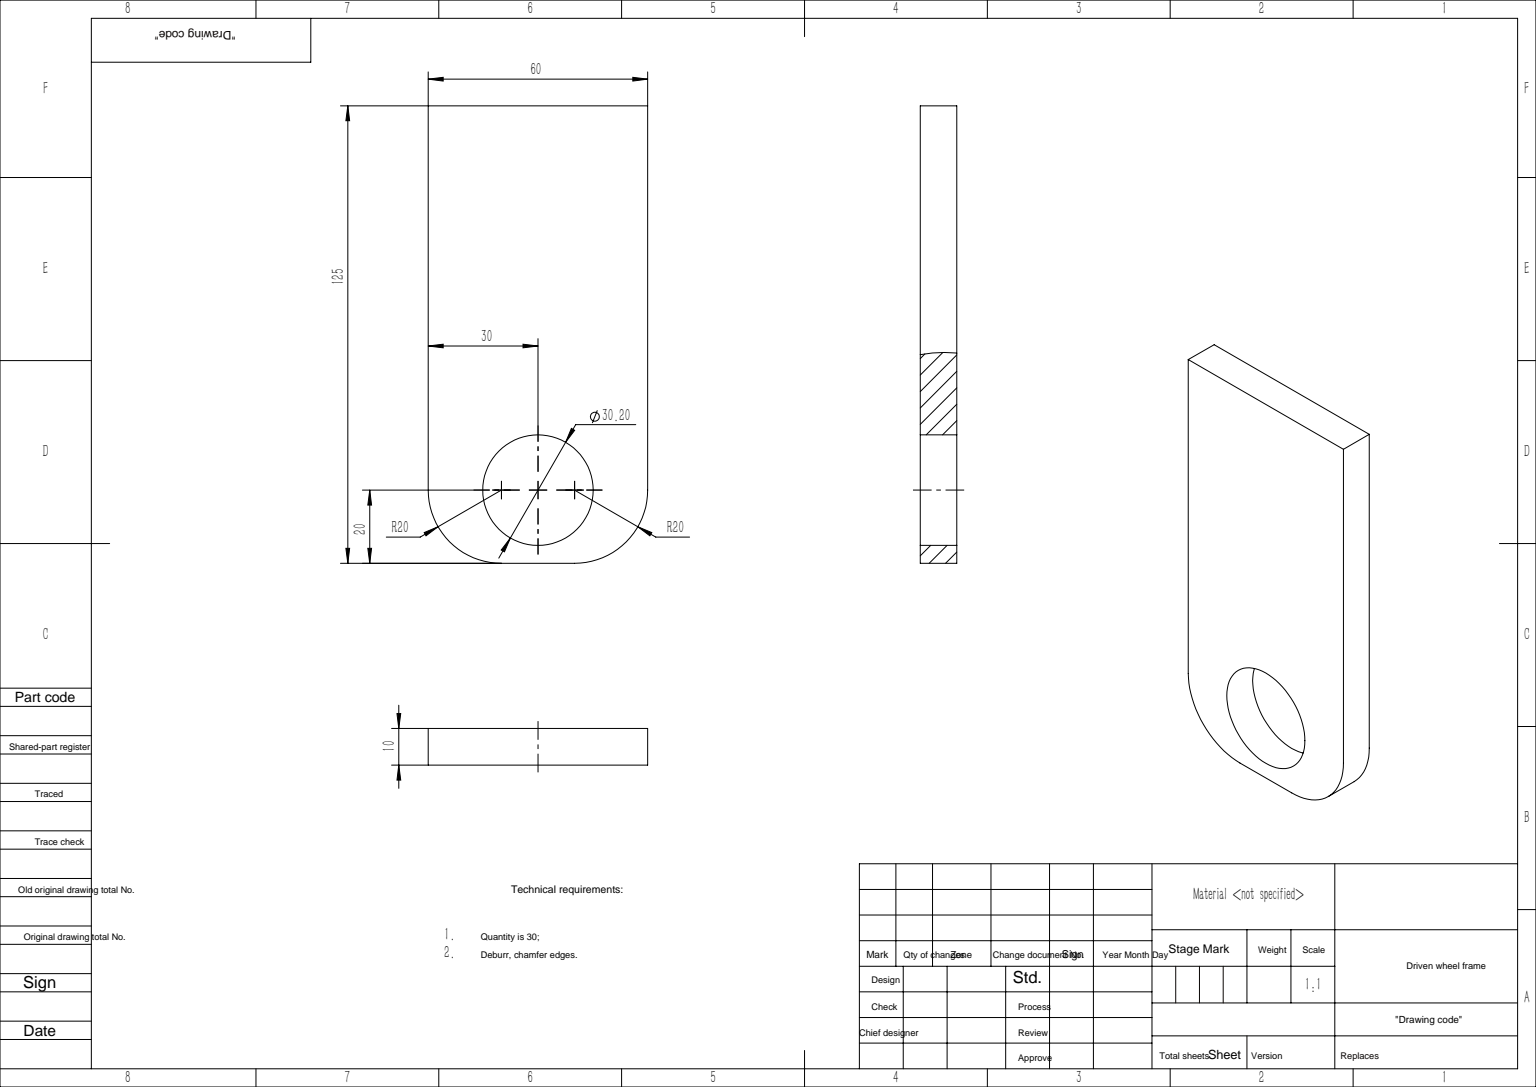
from build123d import *

# Parameters (mm, degrees)
SKETCH_1_W      = 60
SKETCH_1_H      = 125
SKETCH_1_R      = 15.1
EXTRUDE_1_DEPTH = 10
FILLET_1_R      = 20


with BuildPart() as part:
    # 草图1 → 凸台-拉伸1 (new body)
    with BuildSketch(Plane.XY):
        with Locations((0, 42.5)):
            Rectangle(SKETCH_1_W, SKETCH_1_H)
        Circle(SKETCH_1_R, mode=Mode.SUBTRACT)
    extrude(amount=EXTRUDE_1_DEPTH)

    # 圆角1
    fillet_1_edges = [part.edges().sort_by_distance(p)[0] for p in [
        (30, -20, 5),
        (-30, -20, 5),
    ]]
    fillet(fillet_1_edges, radius=FILLET_1_R)


solid = part.part
